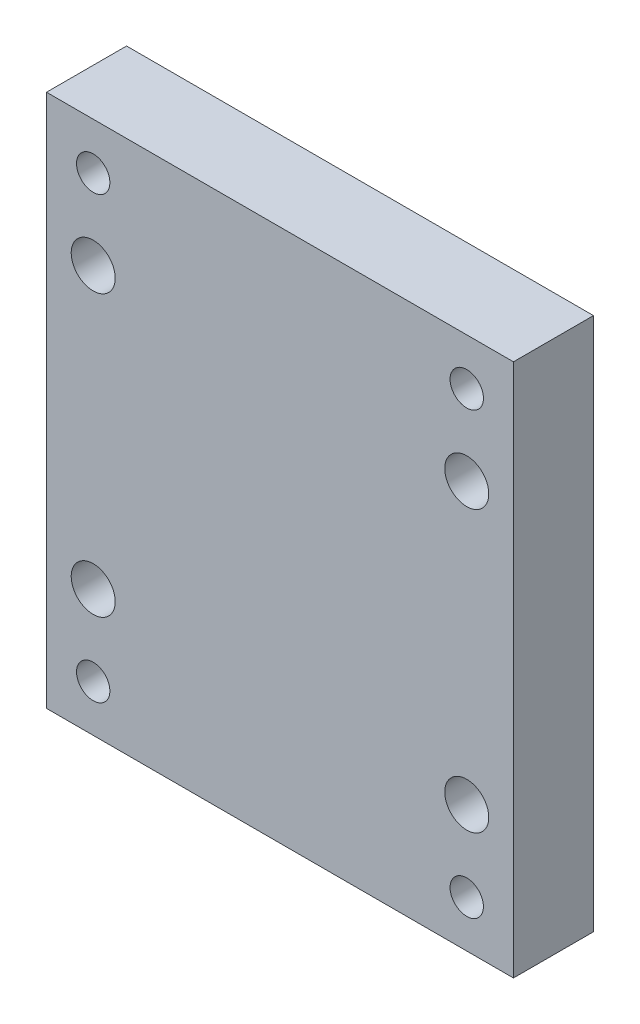
SolidWorks part; units mm, degrees
ref_plane "前视" through (0, 0, 0) normal (0, 0, 1) x (1, 0, 0)
ref_plane "上视" through (0, 0, 0) normal (0, 1, 0) x (1, 0, 0)
ref_plane "右视" through (0, 0, 0) normal (1, 0, 0) x (0, 0, -1)
sketch "草图1" plane through (0, 0, 0) normal (0, 0, 1) x (1, 0, 0)
  line L1 (-35, 40) -> (35, 40)
  line L2 (-35, 40) -> (-35, -40)
  line L3 (-35, -40) -> (35, -40)
  line L4 (35, 40) -> (35, -40)
  line L5 (-35, 40) -> (35, -40) construction
  line L6 (-35, -40) -> (35, 40) construction
  point P0 (0, 0)
  dimension "D1" = 70
  dimension "D2" = 80
extrude "凸台-拉伸1" add sketch "草图1" along normal blind 12
hole_wizard "M6 螺纹孔1" positions "草图3" profile "草图2" tap size "M6" standard "GB" end condition through all
sketch "草图3" plane through (0, 0, 0) normal (0, 0, -1) x (-1, 0, 0)
  point P0 (-28, -33)
  point P3 (-28, 33)
  point P6 (28, 33)
  point P9 (28, -33)
cosmetic thread "孔螺蚊线1" parameters "D2"=6
cosmetic thread "孔螺蚊线2" parameters "D2"=6
cosmetic thread "孔螺蚊线3" parameters "D2"=6
cosmetic thread "孔螺蚊线4" parameters "D2"=6
sketch "草图2" plane through (28, -33, 0) normal (1, 0, 0) x (0, 1, 0)
  line L0 (0, 0) -> (0, 12)
  line L1 (0, 12) -> (2.5, 12)
  line L2 (2.5, 12) -> (2.5, 0)
  line L5 (2.5, 0) -> (0, 0)
  line L11 (0, -6.35) -> (0, 107.95) construction
  dimension "通孔螺纹孔钻头直径" = 5
  dimension "通孔螺纹孔钻头深度" = 12
hole_wizard "M6 六角凹头螺钉的柱形沉头孔1" positions "草图5" profile "草图4" counterbore size "M6" standard "ISO" end condition through all
sketch "草图5" plane through (0, 0, 0) normal (0, 0, -1) x (-1, 0, 0)
  line L0 (0, 0) -> (0, 40) construction
  line L1 (-35, 40) -> (35, 40) construction
  line L4 (-28, 21) -> (-28, -21) construction
  line L7 (-28, 0) -> (0, 0) construction
  line L9 (-35, -40) -> (-35, 40) construction
  point P0 (-28, -21)
  point P2 (-28, 21)
  point P25 (28, -21)
  point P26 (28, 21)
  dimension "D1" = 7
  dimension "D2" = 42
sketch "草图4" plane through (28, -21, 0) normal (1, 0, 0) x (0, 1, 0)
  line L0 (0, 0) -> (0, 12)
  line L1 (0, 12) -> (3.3, 12)
  line L3 (3.3, 12) -> (3.3, 6.4)
  line L4 (3.3, 6.4) -> (5.5, 6.4)
  line L5 (5.5, 6.4) -> (5.5, 0)
  line L7 (5.5, 0) -> (0, 0)
  line L11 (0, -6.35) -> (0, 107.95) construction
  dimension "通孔孔直径" = 6.6
  dimension "通孔孔深度" = 12
  dimension "柱形沉头孔直径" = 11
  dimension "柱形沉头孔深度" = 6.4
sketch "草图6" plane through (0, 0, 0) normal (0, 0, -1) x (-1, 0, 0)
  line L0 (17.5, 35) -> (-17.5, 35) construction
  line L1 (17.5, 32.5) -> (-17.5, 32.5)
  line L2 (17.5, 37.5) -> (-17.5, 37.5)
  line L3 (0, 35) -> (0, 0) construction
  line L4 (-35, 40) -> (35, 40) construction
  arc A0 (17.5, 32.5) -> (17.5, 37.5) centre (17.5, 35) ccw
  arc A1 (-17.5, 37.5) -> (-17.5, 32.5) centre (-17.5, 35) ccw
  point P2 (0, 35)
  dimension "D1" = 5
  dimension "D2" = 2.5
  dimension "D3" = 35
extrude "切除-拉伸1" cut sketch "草图6" against normal blind 2.5
pattern_linear "阵列(线性)1" count 8 spacing 10 along (0, -1, 0) of "切除-拉伸1"
